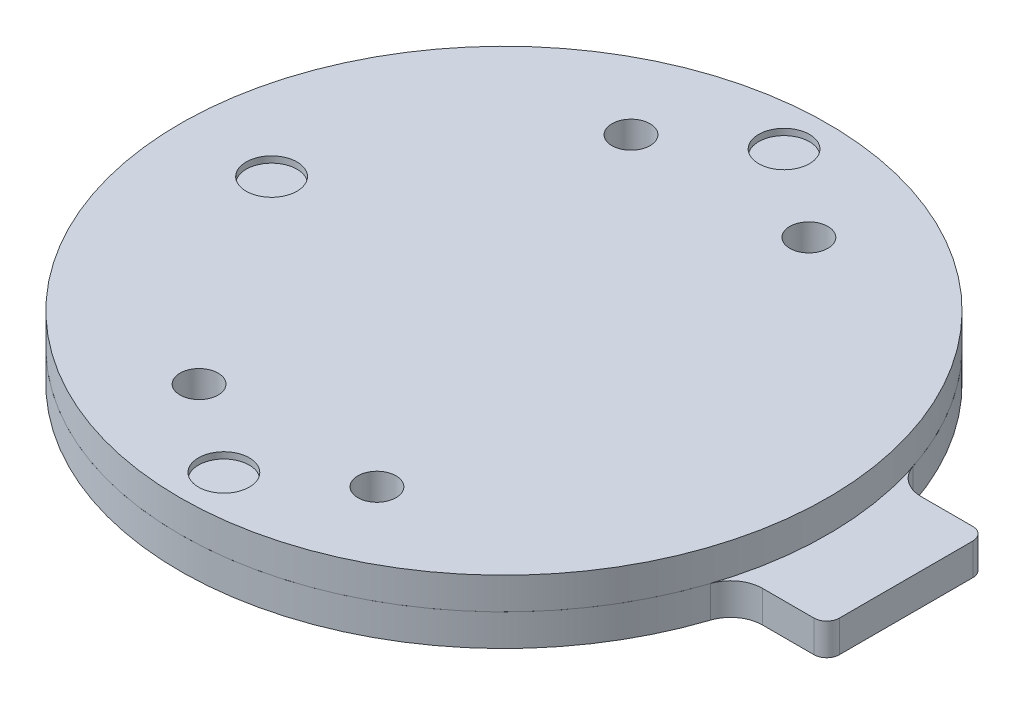
SolidWorks part; units mm, degrees
ref_plane "Front Plane" through (0, 0, 0) normal (0, 0, 1) x (1, 0, 0)
ref_plane "Top Plane" through (0, 0, 0) normal (0, 1, 0) x (1, 0, 0)
ref_plane "Right Plane" through (0, 0, 0) normal (1, 0, 0) x (0, 0, -1)
other "Configuration Table"
sketch "Sketch1" plane through (0, 0, 0) normal (0, 1, 0) x (1, 0, 0)
  circle A0 centre (0, 0) radius 51
  dimension "D1" = 102
extrude "Boss-Extrude1" add sketch "Sketch1" along normal blind 5
sketch "Sketch3" plane through (0, 5, 0) normal (0, 1, 0) x (1, 0, 0)
  line L0 (0, 0) -> (50000, 0) construction
  line L1 (49.4444, 12.5) -> (61.3066, 12.5)
  line L2 (63.3066, 10.5) -> (63.3066, -10.5)
  line L3 (61.3066, -12.5) -> (49.4444, -12.5)
  line L4 (49.4444, 12.5) -> (49.4444, -12.5)
  circle A0 centre (0, 0) radius 51 construction
  arc A1 (61.3066, -12.5) -> (63.3066, -10.5) centre (61.3066, -10.5) ccw
  arc A2 (63.3066, 10.5) -> (61.3066, 12.5) centre (61.3066, 10.5) ccw
  point P11 (63.3066, -12.5)
  point P14 (63.3066, 12.5)
  dimension "D3" = 2
  dimension "D1" = 25
  dimension "D2" = 12.5
extrude "Boss-Extrude2" add sketch "Sketch3" against normal blind 5
fillet "Fillet1" radius 5 2 edges at (49.4444, 2.5, -12.5) (49.4444, 2.5, 12.5)
sketch "Sketch4" plane through (0, 5, 0) normal (0, 1, 0) x (1, 0, 0)
  circle A0 centre (0, 0) radius 51
extrude "Boss-Extrude3" add sketch "Sketch4" along normal blind 5 separate body
sketch "Sketch5" plane through (0, 10, 0) normal (0, 1, 0) x (1, 0, 0)
  line L0 (0, 0) -> (0, 50000) construction
  line L1 (0, 0) -> (-50000, 0) construction
  circle A0 centre (-14, 34) radius 3
  circle A1 centre (14, 34) radius 3
  circle A2 centre (14, -34) radius 3
  circle A3 centre (-14, -34) radius 3
  dimension "D1" = 6
  dimension "D2" = 14
  dimension "D3" = 34
extrude "Cut-Extrude1" cut sketch "Sketch5" against normal through all
sketch "Sketch6" plane through (0, 10, 0) normal (0, 1, 0) x (1, 0, 0)
  line L0 (0, 0) -> (-50000, 0) construction
  circle A0 centre (-36.5849, 0) radius 4
  circle A1 centre (0, -44.095) radius 4
  circle A2 centre (0, 44.095) radius 4
  dimension "D1" = 8
  dimension "D2" = 8
extrude "Cut-Extrude2" cut sketch "Sketch6" against normal blind 1
